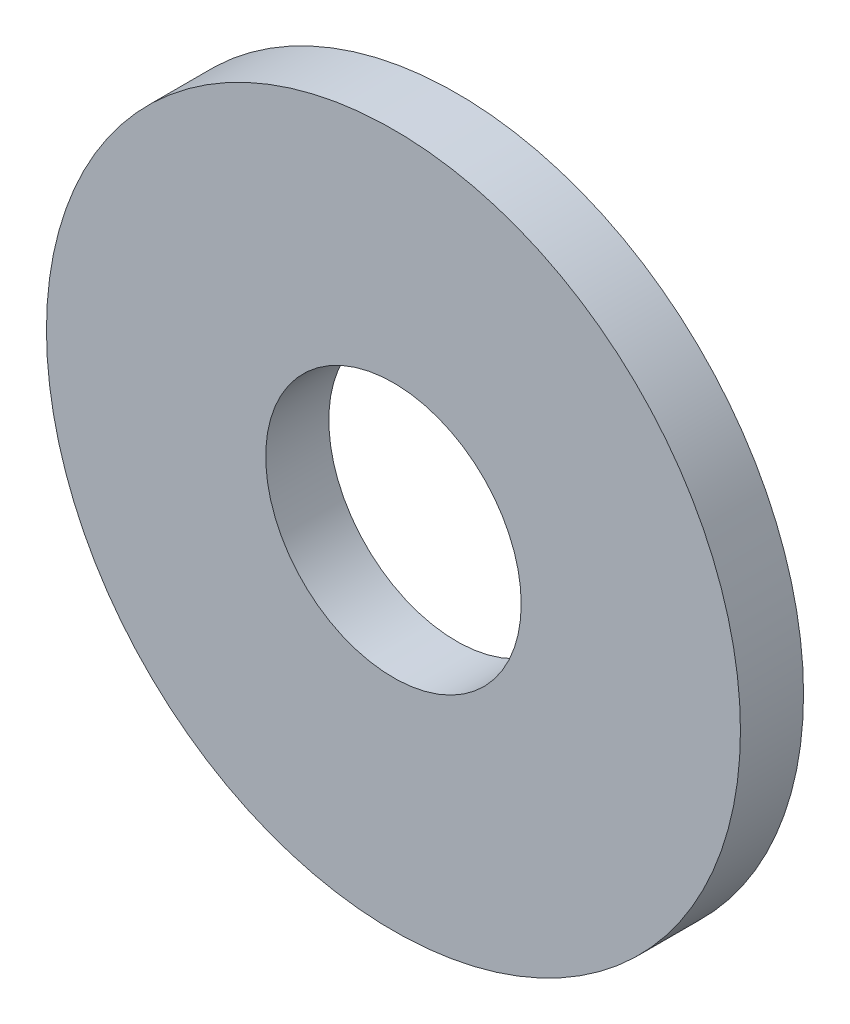
from build123d import *

# Parameters (mm, degrees)
SKETCH_1_R      = 22
SKETCH_1_R_2    = 8.1
EXTRUDE_1_DEPTH = 2


with BuildPart() as part:
    # 草图1 → 凸台-拉伸1 (new, symmetric)
    with BuildSketch(Plane.XY):
        Circle(SKETCH_1_R)
        Circle(SKETCH_1_R_2, mode=Mode.SUBTRACT)
    extrude(amount=EXTRUDE_1_DEPTH, both=True)


solid = part.part
